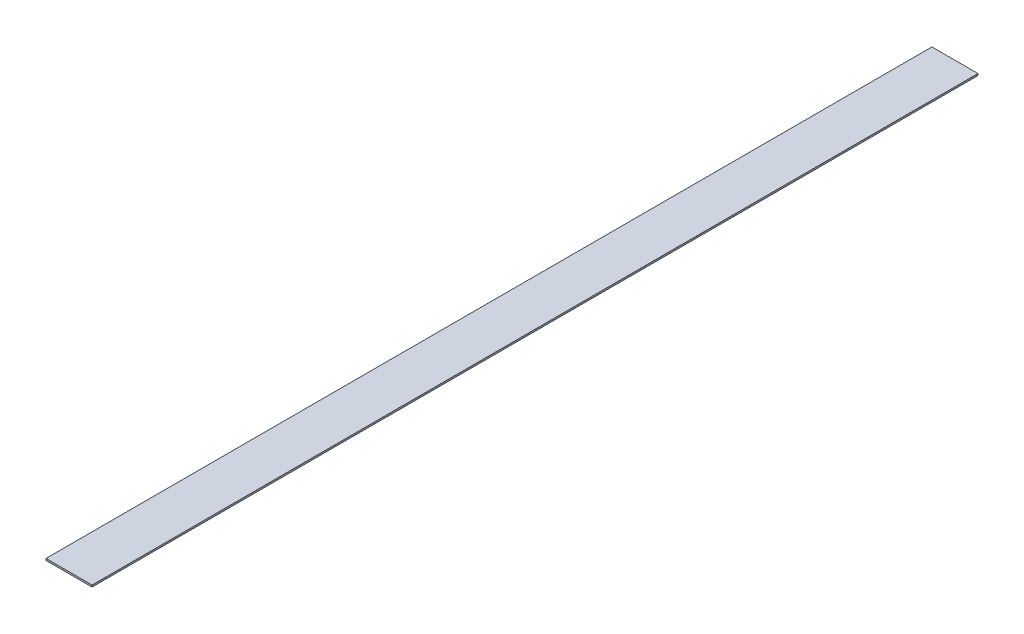
SolidWorks part; units mm, degrees
ref_plane "Front Plane" through (0, 0, 0) normal (0, 0, 1) x (1, 0, 0)
ref_plane "Top Plane" through (0, 0, 0) normal (0, 1, 0) x (1, 0, 0)
ref_plane "Right Plane" through (0, 0, 0) normal (1, 0, 0) x (0, 0, -1)
other "Configuration Table"
sketch "Sketch1" plane through (0, 0, 0) normal (0, 0, 1) x (1, 0, 0)
  line L13 (0, 0) -> (260, 0)
  line L14 (0, 0) -> (0, 10)
  line L15 (0, 10) -> (260, 10)
  line L16 (260, 0) -> (260, 10)
  dimension "D1" = 260
  dimension "D2" = 10
extrude "Boss-Extrude1" add sketch "Sketch1" along normal blind 5000
